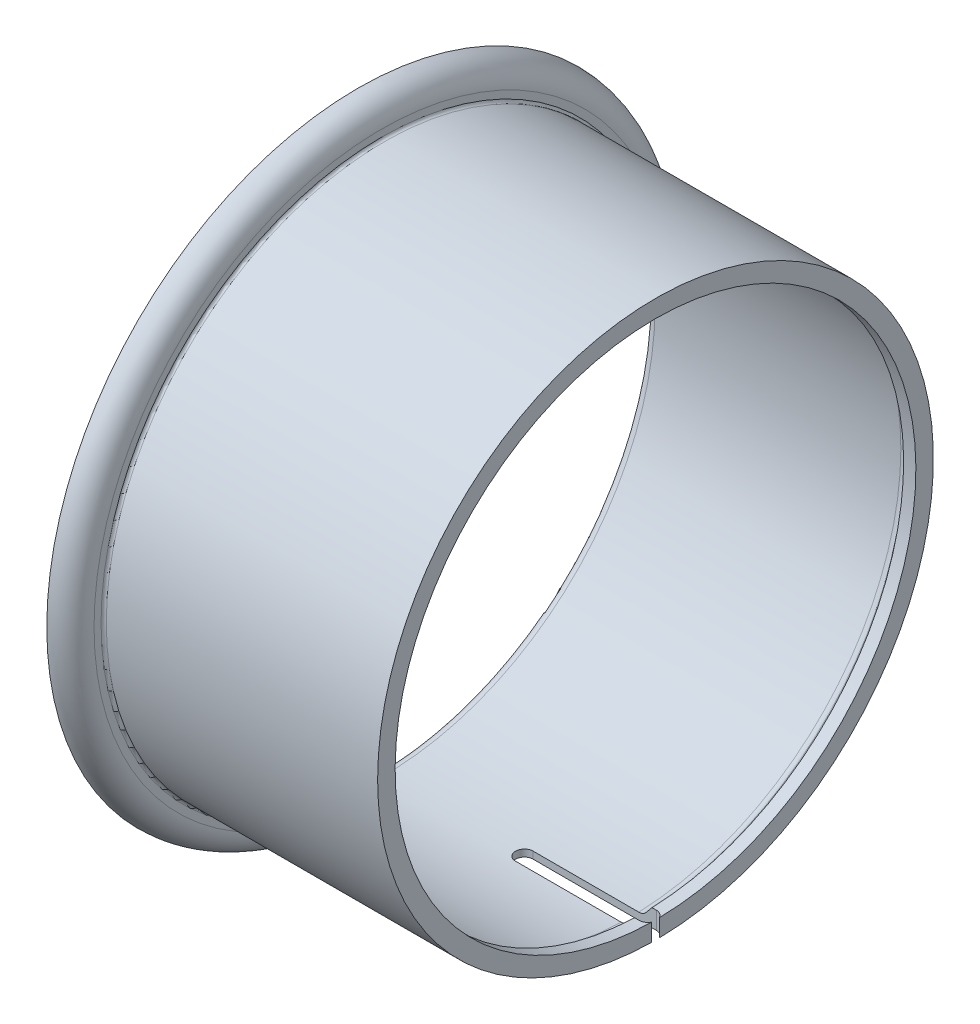
SolidWorks part; units mm, degrees
material "普通碳钢"
ref_plane "前视" through (0, 0, 0) normal (0, 0, 1) x (1, 0, 0)
ref_plane "上视" through (0, 0, 0) normal (0, 1, 0) x (1, 0, 0)
ref_plane "右视" through (0, 0, 0) normal (1, 0, 0) x (0, 0, -1)
sketch "草图1" plane through (0, 0, 0) normal (0, 0, 1) x (1, 0, 0)
  line L0 (-326.8527, 0) -> (318.8021, 0) construction
  line L1 (0, 246.7496) -> (0, -231.4536) construction
  line L2 (19, 328.5) -> (19, 309.5)
  line L3 (27, 328.5) -> (27, 317.5)
  line L5 (27, 317.5) -> (340, 317.5)
  line L6 (19, 309.5) -> (316, 309.5)
  line L7 (316, 309.5) -> (326, 297.5)
  line L8 (326, 297.5) -> (340, 297.5)
  line L9 (340, 297.5) -> (340, 317.5)
  line L10 (0, 355.5) -> (0, 347.5)
  line L11 (9.4362, 317.5) -> (137.1715, 317.5) construction
  line L12 (9.4362, 309.5) -> (137.1715, 309.5) construction
  arc A0 (19, 328.5) -> (0, 347.5) centre (0, 328.5) ccw
  arc A1 (27, 328.5) -> (0, 355.5) centre (0, 328.5) ccw
  dimension "D1" = 38
  dimension "D2" = 54
  dimension "D3" = 635
  dimension "D4" = 8
  dimension "D5" = 11
  dimension "D6" = 340
  dimension "D7" = 20
  dimension "D8" = 14
  dimension "D9" = 316
revolve "旋转1" add sketch "草图1" angle 360 about L0
fillet "圆角2" radius 11 2 edges at (19, 0, 309.5) (316, 0, 309.5)
fillet "圆角3" radius 3 1 edges at (27, 0, 317.5)
sketch "草图2" plane through (0, 0, 0) normal (0, 1, 0) x (1, 0, 0)
  line L0 (310.8479, 0) -> (30, 0) construction
  line L1 (190, 10) -> (331, 10)
  line L2 (190, -10) -> (331, -10)
  line L3 (340, -317.5) -> (340, 317.5) construction
  arc A0 (190, 10) -> (190, -10) centre (190, 0) ccw
  arc A1 (331, -10) -> (331, 10) centre (331, 0) ccw
  dimension "D1" = 20
  dimension "D2" = 141
  dimension "D3" = 9
extrude "切除-拉伸3" cut sketch "草图2" against normal through all
